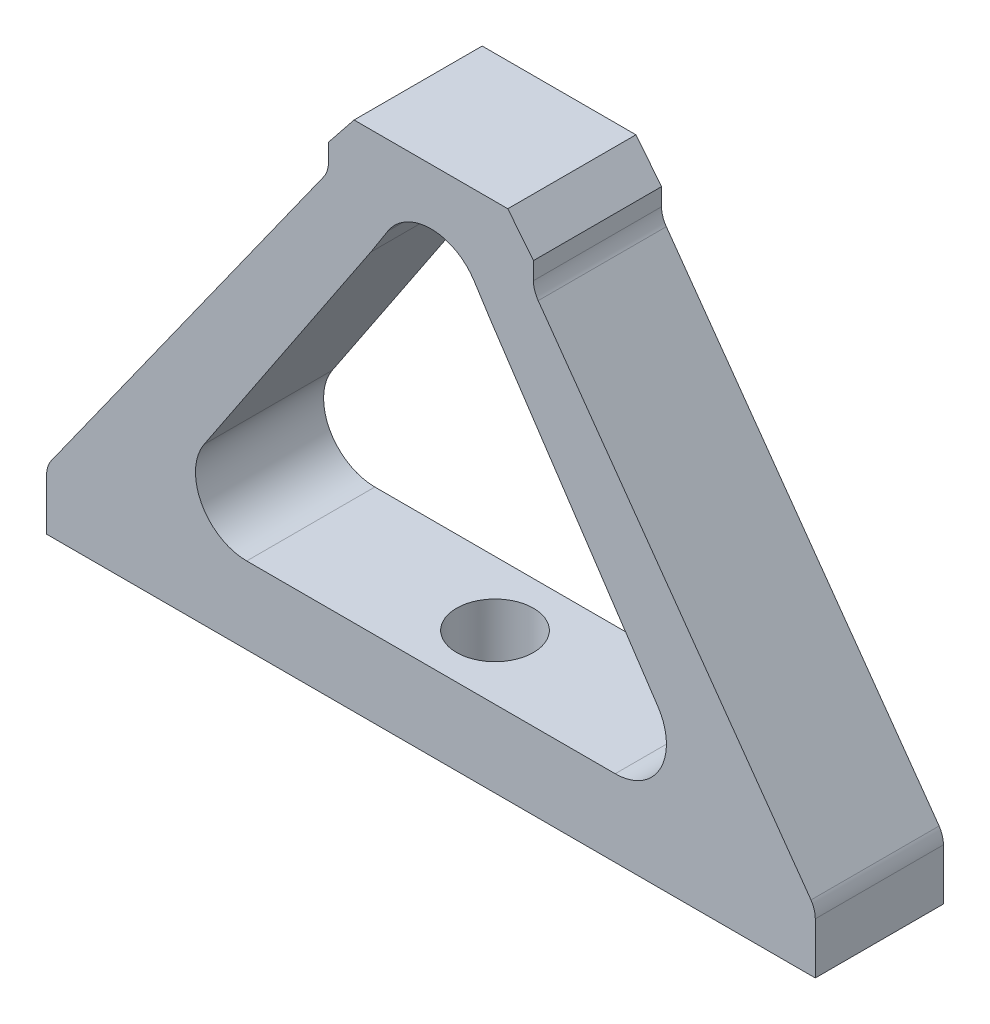
SolidWorks part; units mm, degrees
ref_plane "前视基准面" through (0, 0, 0) normal (0, 0, 1) x (1, 0, 0)
ref_plane "上视基准面" through (0, 0, 0) normal (0, 1, 0) x (1, 0, 0)
ref_plane "右视基准面" through (0, 0, 0) normal (1, 0, 0) x (0, 0, -1)
other "Configuration Table"
sketch "草图1" plane through (0, 0, 0) normal (0, 0, 1) x (1, 0, 0)
  line L0 (-39.891, -1.953) -> (40.677, -1.953) construction
  line L1 (-36.4847, -19.953) -> (23.5153, -19.953)
  line L2 (-24.1922, -7.733) -> (-11.1817, 11.7684)
  line L3 (-36.4847, -19.953) -> (-36.4847, -15.953)
  line L4 (23.5153, -19.953) -> (23.5153, -15.953)
  line L5 (1.8868, 15.0201) -> (23.1792, -14.8433)
  line L6 (-36.1485, -14.843) -> (-14.8563, 15.0201)
  line L7 (-14.4847, 16.1812) -> (-14.4847, 17.5412)
  line L8 (-12.4847, 20.047) -> (-0.4847, 20.047)
  line L9 (-14.4847, 17.5412) -> (-12.4847, 20.047)
  line L10 (-11.1817, 11.7684) -> (-9.8532, 13.8482)
  line L11 (-1.8029, 11.8031) -> (-3.1127, 13.8505)
  line L12 (-1.8029, 11.8031) -> (11.226, -7.7336)
  line L13 (-20.8648, -13.953) -> (7.8981, -13.953)
  line L14 (1.5153, 17.5412) -> (-0.4847, 20.047)
  line L15 (1.5153, 16.1812) -> (1.5153, 17.5412)
  arc A0 (-14.8563, 15.0201) -> (-14.4847, 16.1812) centre (-16.4847, 16.1812) ccw
  arc A1 (1.8868, 15.0201) -> (1.5153, 16.1812) centre (3.5153, 16.1812) cw
  arc A2 (23.5153, -15.953) -> (23.1792, -14.8433) centre (21.5153, -15.953) ccw
  arc A3 (-36.4847, -15.953) -> (-36.1485, -14.843) centre (-34.4847, -15.953) cw
  arc A4 (-3.1127, 13.8505) -> (-9.8532, 13.8482) centre (-6.4822, 11.6949) ccw
  arc A5 (-20.8648, -13.953) -> (-24.1922, -7.733) centre (-20.8648, -9.953) cw
  arc A6 (11.226, -7.7336) -> (7.8981, -13.953) centre (7.8981, -9.953) cw
  point P31 (1.5153, 15.5412)
  dimension "D2" = 2
  dimension "D3" = 4
  dimension "D4" = 4
  dimension "D8" = 2
  dimension "D1" = 60
  dimension "D5" = 18
  dimension "D6" = 4
  dimension "D7" = 40
  dimension "D9" = 4
  dimension "D10" = 12
extrude "凸台-拉伸1" add sketch "草图1" along normal blind 10
ref_plane "基准面1" through (0, -19.953, 0) normal (0, -1, 0) x (-1, 0, 0)
sketch "草图3" plane through (0, -19.953, 0) normal (0, -1, 0) x (1, 0, 0)
  line L0 (-6.4847, 21.7888) -> (-6.4847, -6.7407) construction
  line L1 (-43.8012, 5) -> (28.9587, 5) construction
  line L2 (-36.4847, 10) -> (-36.4847, 0) construction
  line L3 (-36.4847, 0) -> (23.5153, 0) construction
  circle A0 centre (-6.4847, 5) radius 3
  dimension "D1" = 30
  dimension "D2" = 5
extrude "切除-拉伸1" cut sketch "草图3" against normal blind 10
